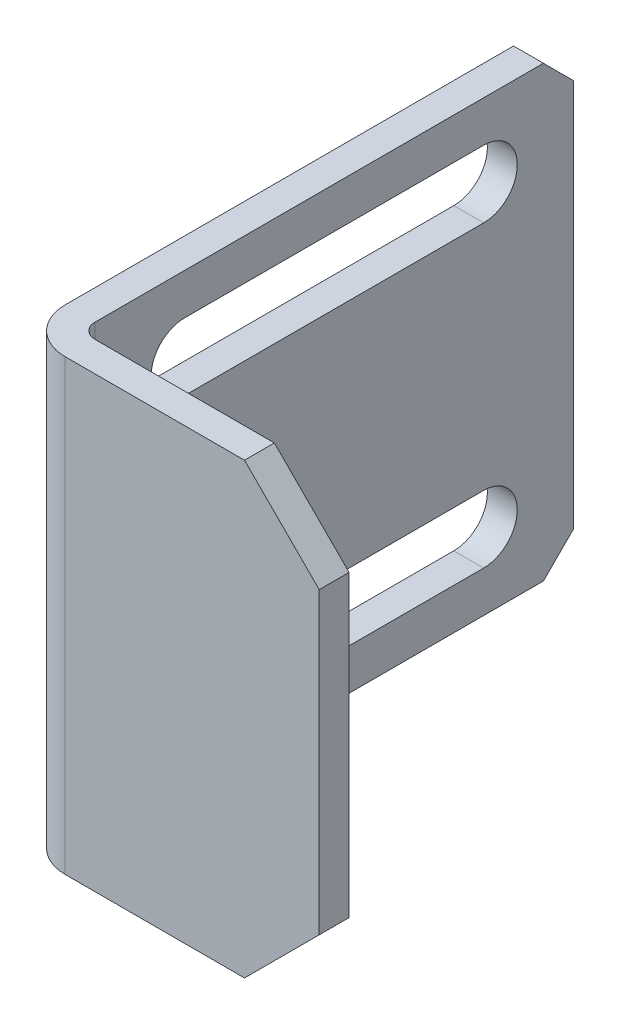
from build123d import *

# Parameters (mm, degrees)
BOSS_EXTRUDE1_DEPTH = 30
SKETCH3_R           = 2.25
CUT_EXTRUDE2_DEPTH  = 10
CHAMFER2_SIZE       = 2
FILLET1_R           = 1
FILLET2_R           = 3
CHAMFER3_SIZE       = 5
CUT_EXTRUDE3_DEPTH  = 10


with BuildPart() as part:
    # Sketch1 → Boss-Extrude1 (new body)
    with BuildSketch(Plane(origin=(0, 0, 0), x_dir=(1, 0, 0), z_dir=(0, 1, 0))):
        Polygon((0, 0), (20, 0), (20, 2), (2, 2), (2, 35), (0, 35), align=None)
    extrude(amount=BOSS_EXTRUDE1_DEPTH)

    # Sketch3 → Cut-Extrude2 (cut)
    with BuildSketch(Plane(origin=(2, 0, 0), x_dir=(0, 0, -1), z_dir=(1, 0, 0))):
        with Locations((29, 25)):
            Circle(SKETCH3_R)
        with Locations((29, 5)):
            Circle(SKETCH3_R)
    extrude(amount=-CUT_EXTRUDE2_DEPTH, mode=Mode.SUBTRACT)

    # Chamfer2
    chamfer2_edges = [part.edges().sort_by_distance(p)[0] for p in [
        (1, 30, -35),
        (1, 0, -35),
    ]]
    chamfer(chamfer2_edges, length=CHAMFER2_SIZE)

    # Fillet1
    fillet1_edges = [part.edges().sort_by_distance(p)[0] for p in [
        (2, 15, -2),
    ]]
    fillet(fillet1_edges, radius=FILLET1_R)

    # Fillet2
    fillet2_edges = [part.edges().sort_by_distance(p)[0] for p in [
        (0, 15, 0),
    ]]
    fillet(fillet2_edges, radius=FILLET2_R)

    # Chamfer3
    chamfer3_edges = [part.edges().sort_by_distance(p)[0] for p in [
        (20, 30, -1),
        (20, 0, -1),
    ]]
    chamfer(chamfer3_edges, length=CHAMFER3_SIZE)

    # Sketch4 → Cut-Extrude3 (cut)
    with BuildSketch(Plane(origin=(2, 0, 0), x_dir=(0, 0, -1), z_dir=(1, 0, 0))):
        with BuildLine():
            Line((29, 2.75), (9, 2.75))
            ThreePointArc((9, 2.75), (6.75, 5), (9, 7.25))
            Line((9, 7.25), (29, 7.25))
            ThreePointArc((29, 7.25), (31.25, 5), (29, 2.75))
        make_face()
        with BuildLine():
            Line((29, 27.25), (9, 27.25))
            ThreePointArc((9, 27.25), (6.75, 25), (9, 22.75))
            Line((9, 22.75), (29, 22.75))
            ThreePointArc((29, 22.75), (31.25, 25), (29, 27.25))
        make_face()
    extrude(amount=-CUT_EXTRUDE3_DEPTH, mode=Mode.SUBTRACT)


solid = part.part
